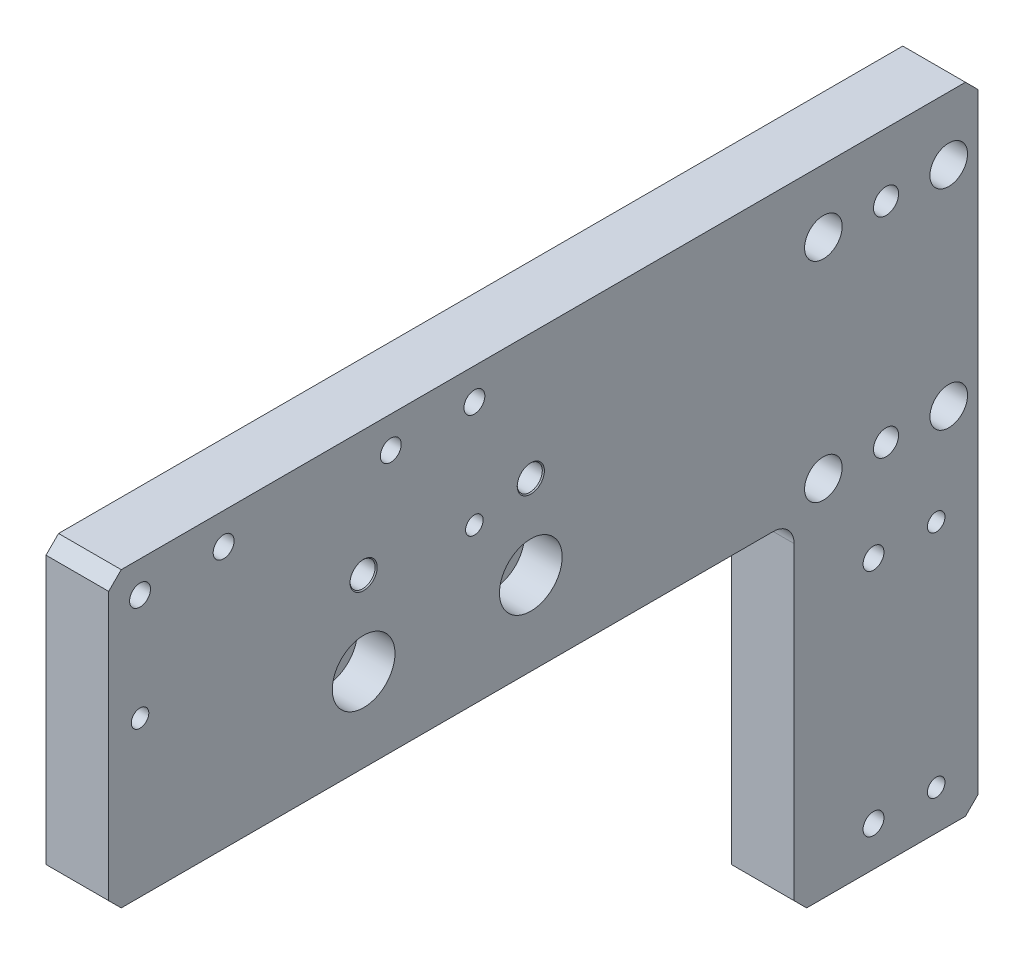
from build123d import *

# Parameters (mm, degrees)
SKETCH1_W                                            = 208
SKETCH1_H                                            = 70.1
BOSS_EXTRUDE1_DEPTH                                  = 15
CBORE_FOR_M8_HEXAGON_SOCKET_HEAD_CAP_SCR_D           = 9
CBORE_FOR_M8_HEXAGON_SOCKET_HEAD_CAP_SCR_CBORE_D     = 15
CBORE_FOR_M8_HEXAGON_SOCKET_HEAD_CAP_SCR_CBORE_DEPTH = 9
F_6_0MM_BLIND_HOLE_1_AT_2_COUNT                      = 2
F_6_0MM_BLIND_HOLE_1_AT_2_PITCH                      = 40
SKETCH6_W                                            = 15
SKETCH6_H                                            = 44
BOSS_EXTRUDE2_DEPTH                                  = 82
M5_TAPPED_HOLE1_D                                    = 4.2
M5_TAPPED_HOLE1_DEPTH                                = 12.4
M5_TAPPED_HOLE1_TIP                                  = 1.2618073
F_5_0MM_BLIND_HOLE_1_D                               = 5
F_5_0MM_BLIND_HOLE_1_DEPTH                           = 8
F_5_0MM_BLIND_HOLE_1_TIP                             = 1.502151548
M6_TAPPED_HOLE1_D                                    = 5
M6_TAPPED_HOLE1_DEPTH                                = 15
M6_TAPPED_HOLE1_TIP                                  = 1.502151548
F_5_0MM_BLIND_HOLE_2_D                               = 5
F_5_0MM_BLIND_HOLE_2_DEPTH                           = 8
F_5_0MM_BLIND_HOLE_2_TIP                             = 1.502151548
M5_TAPPED_HOLE2_D                                    = 4.2
M5_TAPPED_HOLE2_DEPTH                                = 12.4
M5_TAPPED_HOLE2_TIP                                  = 1.2618073
M8_CLEARANCE_HOLE1_D                                 = 9
F_6_0MM_BLIND_HOLE_2_D                               = 6
FILLET1_R                                            = 5
CHAMFER1_SIZE                                        = 3


with BuildPart() as part:
    # Sketch1 → Boss-Extrude1 (new body)
    with BuildSketch(Plane(origin=(0, 0, 0), x_dir=(0, 0, -1), z_dir=(1, 0, 0))):
        Rectangle(SKETCH1_W, SKETCH1_H)
    extrude(amount=BOSS_EXTRUDE1_DEPTH)

    # CBORE for M8 Hexagon socket head cap screws1 (through all)
    with Locations(Plane(origin=(15, 0, 0), x_dir=(0, 0, -1), z_dir=(1, 0, 0))):
        with Locations((-43, -15.05), (-3, -15.05)):
            CounterBoreHole(CBORE_FOR_M8_HEXAGON_SOCKET_HEAD_CAP_SCR_D / 2, CBORE_FOR_M8_HEXAGON_SOCKET_HEAD_CAP_SCR_CBORE_D / 2, CBORE_FOR_M8_HEXAGON_SOCKET_HEAD_CAP_SCR_CBORE_DEPTH)

    # Sketch5 → Ø6.0mm blind hole 1 (revolve, cut)
    with BuildSketch(Plane(origin=(15, 4.95, 43), x_dir=(0, 0, -1), z_dir=(0, 1, 0))):
        Polygon((0, 0), (0, 15), (3.25, 15), (3, 14.75), (3, 0.25), (3.25, 0), align=None)
    f_6_0mm_blind_hole_1 = revolve(axis=Axis((21.35, 4.95, 43), (-1, 0, 0)), mode=Mode.SUBTRACT)

    # Ø6.0mm blind hole 1 at 2: Ø6.0mm blind hole 1 ×2
    with Locations(*[(0, 0, -i * F_6_0MM_BLIND_HOLE_1_AT_2_PITCH) for i in range(1, F_6_0MM_BLIND_HOLE_1_AT_2_COUNT)]):
        add(f_6_0mm_blind_hole_1, mode=Mode.SUBTRACT)

    # Sketch6 → Boss-Extrude2 (add)
    with BuildSketch(Plane.XZ.offset(35.05)):
        with Locations((7.5, -82)):
            Rectangle(SKETCH6_W, SKETCH6_H)
    extrude(amount=BOSS_EXTRUDE2_DEPTH)

    # M5 Tapped Hole1
    with Locations(Plane(origin=(15, 0, 0), x_dir=(0, 0, -1), z_dir=(1, 0, 0))):
        with Locations((94, -107.55), (94, -52.55)):
            Hole(M5_TAPPED_HOLE1_D / 2, depth=M5_TAPPED_HOLE1_DEPTH)
            with Locations((0, 0, -(M5_TAPPED_HOLE1_DEPTH + M5_TAPPED_HOLE1_TIP / 2))):  # 118° drill point
                Cone(0, M5_TAPPED_HOLE1_D / 2, M5_TAPPED_HOLE1_TIP, mode=Mode.SUBTRACT)

    # Ø5.0mm blind hole 1
    with Locations(Plane(origin=(15, 0, 0), x_dir=(0, 0, -1), z_dir=(1, 0, 0))):
        with Locations((79, -52.55), (79, -107.55)):
            Hole(F_5_0MM_BLIND_HOLE_1_D / 2, depth=F_5_0MM_BLIND_HOLE_1_DEPTH)
            with Locations((0, 0, -(F_5_0MM_BLIND_HOLE_1_DEPTH + F_5_0MM_BLIND_HOLE_1_TIP / 2))):  # 118° drill point
                Cone(0, F_5_0MM_BLIND_HOLE_1_D / 2, F_5_0MM_BLIND_HOLE_1_TIP, mode=Mode.SUBTRACT)

    # M6 Tapped Hole1
    with Locations(Plane(origin=(15, 0, 0), x_dir=(0, 0, -1), z_dir=(1, 0, 0))):
        with Locations((-76.5, 27.55), (-36.5, 27.55)):
            Hole(M6_TAPPED_HOLE1_D / 2, depth=M6_TAPPED_HOLE1_DEPTH)
            with Locations((0, 0, -(M6_TAPPED_HOLE1_DEPTH + M6_TAPPED_HOLE1_TIP / 2))):  # 118° drill point
                Cone(0, M6_TAPPED_HOLE1_D / 2, M6_TAPPED_HOLE1_TIP, mode=Mode.SUBTRACT)

    # Ø5.0mm blind hole 2
    with Locations(Plane(origin=(15, 0, 0), x_dir=(0, 0, -1), z_dir=(1, 0, 0))):
        with Locations((-96.5, 27.55), (-16.5, 27.55)):
            Hole(F_5_0MM_BLIND_HOLE_2_D / 2, depth=F_5_0MM_BLIND_HOLE_2_DEPTH)
            with Locations((0, 0, -(F_5_0MM_BLIND_HOLE_2_DEPTH + F_5_0MM_BLIND_HOLE_2_TIP / 2))):  # 118° drill point
                Cone(0, F_5_0MM_BLIND_HOLE_2_D / 2, F_5_0MM_BLIND_HOLE_2_TIP, mode=Mode.SUBTRACT)

    # M5 Tapped Hole2
    with Locations(Plane(origin=(15, 0, 0), x_dir=(0, 0, -1), z_dir=(1, 0, 0))):
        with Locations((-96.5, 2.05), (-16.5, 2.05)):
            Hole(M5_TAPPED_HOLE2_D / 2, depth=M5_TAPPED_HOLE2_DEPTH)
            with Locations((0, 0, -(M5_TAPPED_HOLE2_DEPTH + M5_TAPPED_HOLE2_TIP / 2))):  # 118° drill point
                Cone(0, M5_TAPPED_HOLE2_D / 2, M5_TAPPED_HOLE2_TIP, mode=Mode.SUBTRACT)

    # M8 Clearance Hole1 (through all)
    with Locations(Plane(origin=(15, 0, 0), x_dir=(0, 0, -1), z_dir=(1, 0, 0))):
        with Locations((67, -30.05), (97, -30.05), (67, 19.95), (97, 19.95)):
            Hole(M8_CLEARANCE_HOLE1_D / 2)

    # Ø6.0mm blind hole 2 (through all)
    with Locations(Plane(origin=(15, 0, 0), x_dir=(0, 0, -1), z_dir=(1, 0, 0))):
        with Locations((82, -30.05), (82, 19.95)):
            Hole(F_6_0MM_BLIND_HOLE_2_D / 2)

    # Fillet1
    fillet1_edges = [part.edges().sort_by_distance(p)[0] for p in [
        (7.5, -35.05, -60),
    ]]
    fillet(fillet1_edges, radius=FILLET1_R)

    # Chamfer1
    chamfer1_edges = [part.edges().sort_by_distance(p)[0] for p in [
        (7.5, -117.05, -104),
        (7.5, -117.05, -60),
        (7.5, -35.05, 104),
        (7.5, 35.05, 104),
        (7.5, 35.05, -104),
    ]]
    chamfer(chamfer1_edges, length=CHAMFER1_SIZE)


solid = part.part
